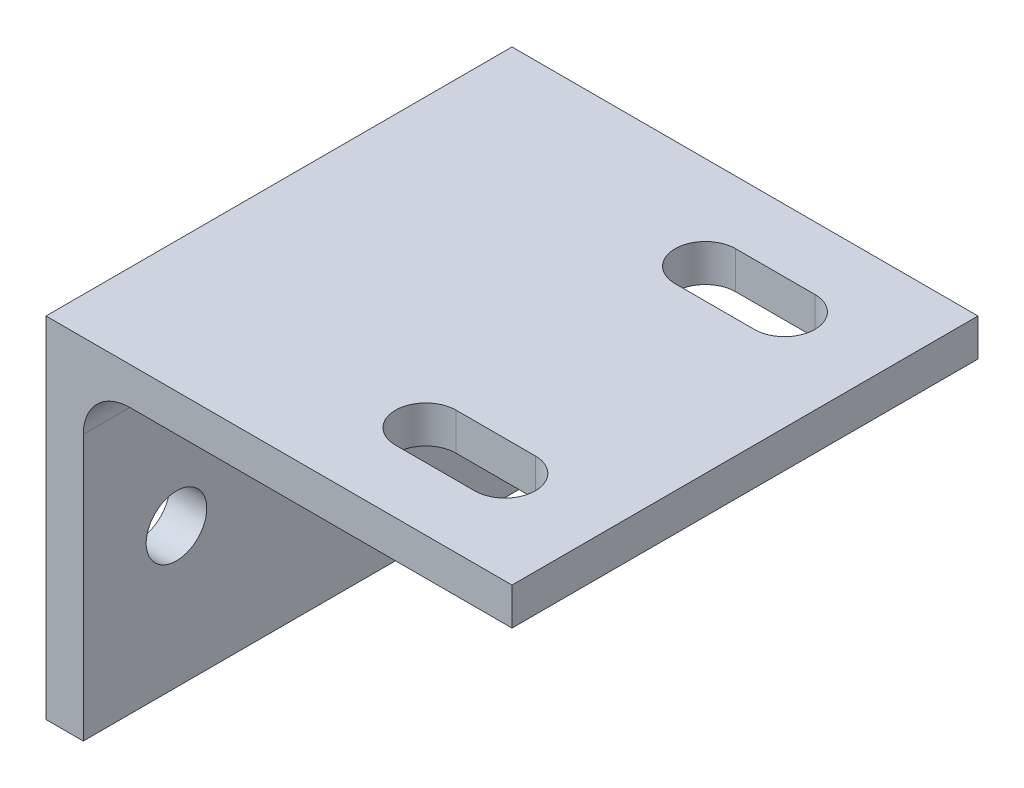
SolidWorks part; units mm, degrees
material "1023 碳钢板 (SS)"
ref_plane "前视基准面" through (0, 0, 0) normal (0, 0, 1) x (1, 0, 0)
ref_plane "上视基准面" through (0, 0, 0) normal (0, 1, 0) x (1, 0, 0)
ref_plane "右视基准面" through (0, 0, 0) normal (1, 0, 0) x (0, 0, -1)
sketch "草图1" plane through (0, 0, 0) normal (0, 0, 1) x (1, 0, 0)
  line L0 (0, 0) -> (-100, 0)
  line L1 (-100, 0) -> (-100, -75)
  line L2 (0, -8) -> (-92, -8)
  line L3 (-92, -8) -> (-92, -75)
  line L4 (0, 0) -> (0, -8)
  line L5 (-92, -75) -> (-100, -75)
  dimension "D1" = 100
  dimension "D2" = 75
  dimension "D3" = 8
extrude "凸台-拉伸1" add sketch "草图1" along normal blind 100
sketch "草图2" plane through (0, 0, 0) normal (0, 1, 0) x (1, 0, 0)
  line L0 (-38.5, -20) -> (-21.5, -20) construction
  line L1 (-38.5, -13.5) -> (-21.5, -13.5)
  line L2 (-38.5, -26.5) -> (-21.5, -26.5)
  line L3 (-38.5, -80) -> (-21.5, -80) construction
  line L4 (-38.5, -73.5) -> (-21.5, -73.5)
  line L5 (-38.5, -86.5) -> (-21.5, -86.5)
  line L6 (0, -100) -> (0, 0) construction
  line L7 (-100, -100) -> (-100, 0) construction
  arc A0 (-38.5, -13.5) -> (-38.5, -26.5) centre (-38.5, -20) ccw
  arc A1 (-21.5, -26.5) -> (-21.5, -13.5) centre (-21.5, -20) ccw
  arc A2 (-38.5, -73.5) -> (-38.5, -86.5) centre (-38.5, -80) ccw
  arc A3 (-21.5, -86.5) -> (-21.5, -73.5) centre (-21.5, -80) ccw
  point P2 (-30, -20)
  point P7 (-30, -80)
  point P16 (0, -50)
  dimension "D1" = 6.5
  dimension "D4" = 61.5
  dimension "D2" = 60
  dimension "D3" = 30
  dimension "D5" = 17
extrude "切除-拉伸1" cut sketch "草图2" against normal blind 100
sketch "草图3" plane through (-92, 0, 0) normal (1, 0, 0) x (0, 0, -1)
  line L0 (-100, 0) -> (0, 0) construction
  line L1 (-100, -75) -> (-100, -8) construction
  circle A0 centre (-80, -45) radius 6.5
  circle A1 centre (-20, -45) radius 6.5
  dimension "D2" = 60
  dimension "D4" = 13
  dimension "D1" = 45
  dimension "D3" = 20
extrude "切除-拉伸2" cut sketch "草图3" against normal blind 100
fillet "圆角1" radius 10 1 edges at (-92, -8, 50)
